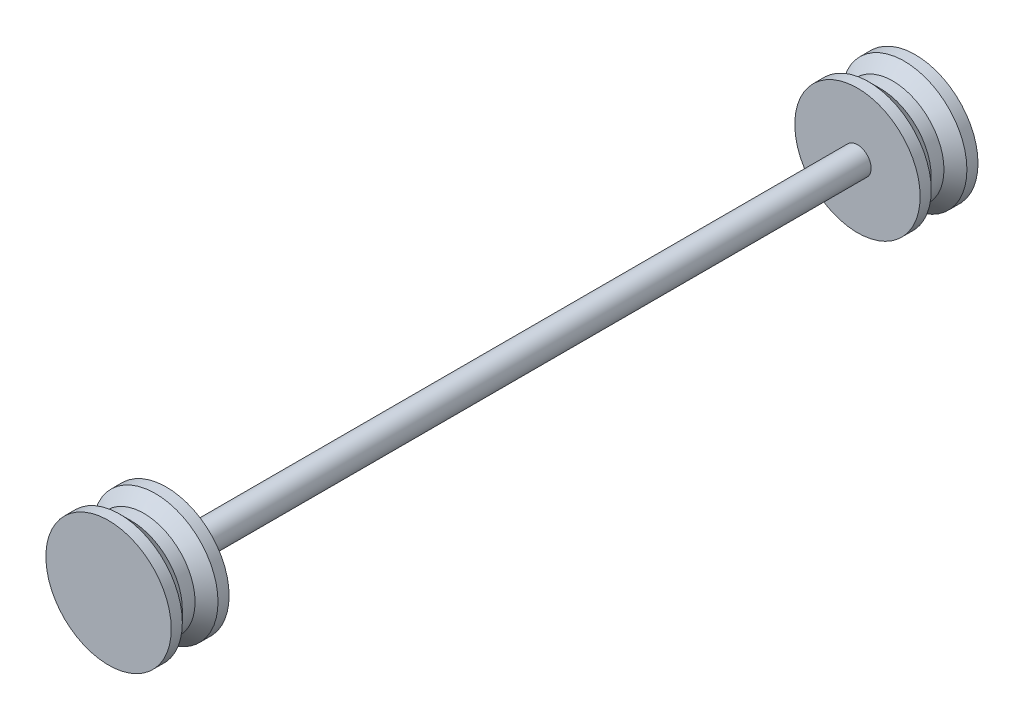
from build123d import *

# Parameters (mm, degrees)
SKETCH1_R           = 1.179493096
BOSS_EXTRUDE1_DEPTH = 59.73181499
SKETCH2_R           = 5.417808654
BOSS_EXTRUDE2_DEPTH = 5


with BuildPart() as part:
    # Sketch1 → Boss-Extrude1 (new body)
    with BuildSketch(Plane.XY):
        with Locations((-29.791335202, -6.219759883)):
            Circle(SKETCH1_R)
    extrude(amount=-BOSS_EXTRUDE1_DEPTH)

    # Sketch2 → Boss-Extrude2 (add)
    with BuildSketch(Plane.XY):
        with Locations((-29.791335202, -6.219759883)):
            Circle(SKETCH2_R)
    boss_extrude2 = extrude(amount=BOSS_EXTRUDE2_DEPTH)

    # Mirror1: Boss-Extrude2 across plane
    add(boss_extrude2.mirror(Plane.XY.offset(-29.865907495)))

    # Sketch4 → Cut-Revolve2 (revolve, cut)
    with BuildSketch(Plane(origin=(0, -6.219759883, 0), x_dir=(0, 0, -1), z_dir=(0, 1, 0)), mode=Mode.PRIVATE) as cut_revolve2_sk:
        Polygon((-4.042100794, 35.209143856), (-3.05057693, 34.217619991), (-1.94942307, 34.217619991), (-0.957899206, 35.209143856), align=None)
        Polygon((60.689714196, 35.209143856), (61.68123806, 34.217619991), (62.78239192, 34.217619991), (63.773915784, 35.209143856), align=None)
    revolve(cut_revolve2_sk.sketch.rotate(Axis((-29.791335202, -6.219759883, 5), (0, 0, -1)), 180), axis=Axis((-29.791335202, -6.219759883, 5), (0, 0, -1)), mode=Mode.SUBTRACT)


solid = part.part
